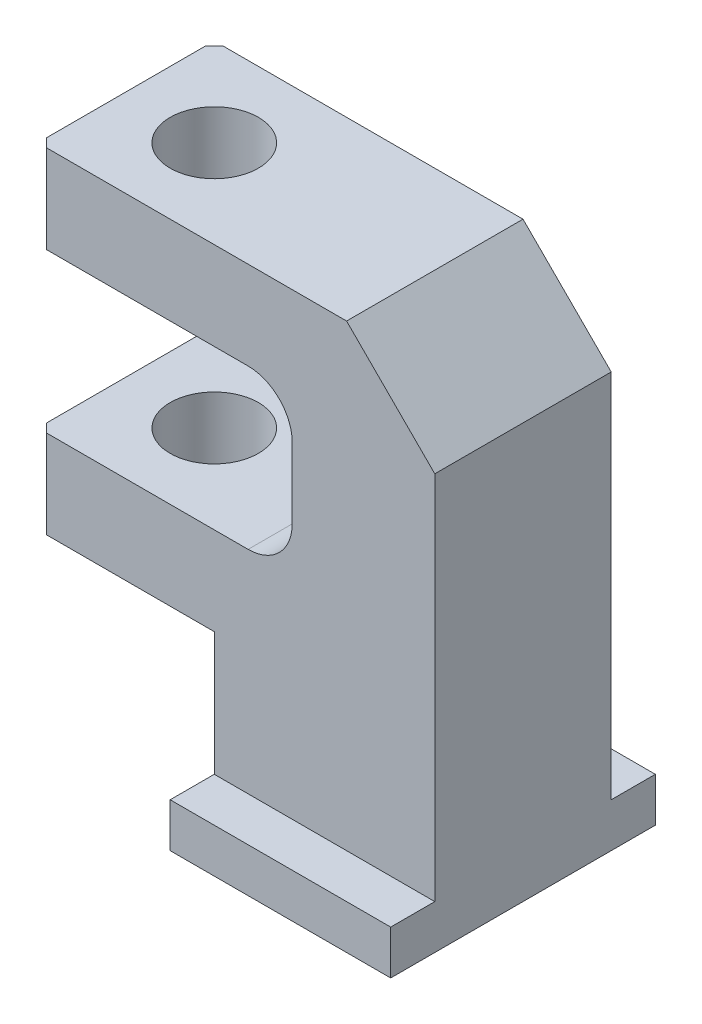
SolidWorks part; units mm, degrees
ref_plane "前视基准面" through (0, 0, 0) normal (0, 0, 1) x (1, 0, 0)
ref_plane "上视基准面" through (0, 0, 0) normal (0, 1, 0) x (1, 0, 0)
ref_plane "右视基准面" through (0, 0, 0) normal (1, 0, 0) x (0, 0, -1)
ref_plane "基准面4" through (17.1454, 0, 0) normal (1, 0, 0) x (0, 0, -1)
sketch "草图1" plane through (17.1454, 0, 0) normal (1, 0, 0) x (0, 0, -1)
  line L0 (15, 57) -> (-15, 57)
  line L1 (-15, 57) -> (-15, 0)
  line L2 (-15, 0) -> (15, 0)
  line L3 (15, 0) -> (15, 57)
extrude "凸台-拉伸1" add sketch "草图1" against normal blind 25
sketch "草图2" plane through (17.1454, 0, 0) normal (1, 0, 0) x (0, 0, -1)
  line L0 (-15, 5) -> (-10, 5)
  line L1 (-10, 5) -> (-10, 57)
  line L2 (-10, 57) -> (-15, 57)
  line L3 (-15, 57) -> (-15, 5)
extrude "切除-拉伸1" cut sketch "草图2" against normal through all
sketch "草图3" plane through (17.1454, 0, 0) normal (1, 0, 0) x (0, 0, -1)
  line L0 (10, 5) -> (15, 5)
  line L1 (15, 5) -> (15, 57)
  line L2 (15, 57) -> (10, 57)
  line L3 (10, 57) -> (10, 5)
extrude "切除-拉伸2" cut sketch "草图3" against normal through all
sketch "草图4" plane through (-7.8546, 0, 0) normal (-1, 0, 0) x (0, 0, 1)
  line L0 (-10, 57) -> (10, 57)
  line L1 (10, 57) -> (10, 19)
  line L2 (10, 19) -> (-10, 19)
  line L3 (-10, 19) -> (-10, 57)
extrude "凸台-拉伸2" add sketch "草图4" along normal blind 20
sketch "草图5" plane through (0, 0, 10) normal (0, 0, 1) x (1, 0, 0)
  line L0 (-27.8546, 47) -> (-27.8546, 29)
  line L1 (-27.8546, 29) -> (0.9816, 29)
  line L2 (0.9816, 29) -> (0.9816, 47)
  line L3 (0.9816, 47) -> (-27.8546, 47)
extrude "切除-拉伸3" cut sketch "草图5" against normal through all
hole_wizard "Ø10.0 (10) 直径孔1" positions "草图7" profile "草图6" hole size "Ø10.0" standard "ANSI Metric"
sketch "草图7" plane through (0, 47, 0) normal (0, -1, 0) x (-1, 0, 0)
  point P0 (17.8546, 0)
sketch "草图6" plane through (-17.8546, 47, 0) normal (1, 0, 0) x (0, 0, -1)
  line L0 (0, 0) -> (0, 10)
  line L1 (0, 10) -> (5, 10)
  line L2 (5, 10) -> (5, 0)
  line L5 (5, 0) -> (0, 0)
  line L11 (0, -6.35) -> (0, 107.95) construction
  dimension "通孔孔直径" = 10
  dimension "通孔孔深度" = 10
hole_wizard "Ø10.0 (10) 直径孔2" positions "草图9" profile "草图8" hole size "Ø10.0" standard "ANSI Metric"
sketch "草图9" plane through (0, 19, 0) normal (0, -1, 0) x (-1, 0, 0)
  point P0 (17.8546, 0)
sketch "草图8" plane through (-17.8546, 19, 0) normal (1, 0, 0) x (0, 0, -1)
  line L0 (0, 0) -> (0, 38)
  line L1 (0, 38) -> (5, 38)
  line L2 (5, 38) -> (5, 0)
  line L5 (5, 0) -> (0, 0)
  line L11 (0, -6.35) -> (0, 107.95) construction
  dimension "通孔孔直径" = 10
  dimension "通孔孔深度" = 38
hole_wizard "Ø5.0 (5) 直径孔1" positions "草图11" profile "草图10" hole size "Ø5.0" standard "ANSI Metric"
sketch "草图11" plane through (0, 0, 0) normal (0, -1, 0) x (-1, 0, 0)
  point P0 (2.8546, 0)
  point P1 (-12.1454, 0)
sketch "草图10" plane through (-2.8546, 0, 0) normal (1, 0, 0) x (0, 0, -1)
  line L0 (0, 0) -> (0, 18.5022)
  line L1 (0, 18.5022) -> (2.5, 17)
  line L2 (2.5, 17) -> (2.5, 0)
  line L5 (2.5, 0) -> (0, 0)
  line L10 (0, 18.5022) -> (-2.5, 17) construction
  line L11 (0, -6.35) -> (0, 107.95) construction
  dimension "孔直径" = 5
  dimension "孔深度" = 17
  dimension "导头角度" = 118
chamfer "倒角1" distance 1 angle 45 4 edges at (-27.8546, 24, -10) (-27.8546, 52, -10) (-27.8546, 24, 10) (-27.8546, 52, 10)
chamfer "倒角2" distance 10 angle 45 1 edges at (17.1454, 57, 0)
fillet "圆角1" radius 5 2 edges at (0.9816, 29, 0) (0.9816, 47, 0)
